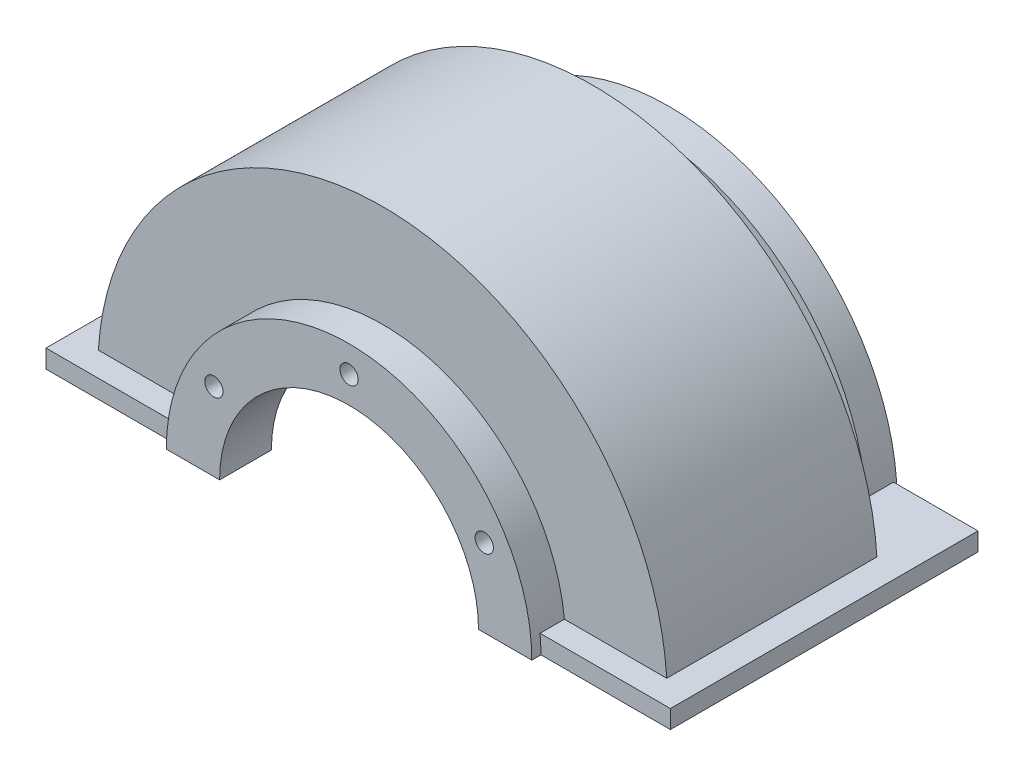
SolidWorks part; units mm, degrees
ref_plane "Front Plane" through (0, 0, 0) normal (0, 0, 1) x (1, 0, 0)
ref_plane "Top Plane" through (0, 0, 0) normal (0, 1, 0) x (1, 0, 0)
ref_plane "Right Plane" through (0, 0, 0) normal (1, 0, 0) x (0, 0, -1)
ref_plane "Plane1" through (0, 0, -358.693) normal (0, 0, -1) x (-1, 0, 0)
sketch "Sketch1" plane through (0, 0, -358.693) normal (0, 0, -1) x (-1, 0, 0)
  line L0 (-707.8452, 246.744) -> (-726.2306, 246.744)
  line L1 (-726.2306, 246.744) -> (-726.2306, 234.744)
  line L2 (-726.2306, 234.744) -> (-316.2306, 234.744)
  line L3 (-316.2306, 234.744) -> (-316.2306, 246.744)
  line L4 (-316.2306, 246.744) -> (-334.6161, 246.744)
  arc A0 (-334.6161, 246.744) -> (-707.8452, 246.744) centre (-521.2306, 234.744) ccw
  dimension "D1" = 187
  dimension "D2" = 18.3854
  dimension "D3" = 205
  dimension "D5" = 410
extrude "Boss-Extrude1" add sketch "Sketch1" against normal blind 202
sketch "Sketch2" plane through (0, 0, -156.693) normal (0, 0, 1) x (1, 0, 0)
  line L0 (640.6291, 246.744) -> (707.8452, 246.744)
  line L1 (334.6161, 246.744) -> (401.8322, 246.744)
  line L2 (316.2306, 234.744) -> (316.2306, 246.744) construction
  line L3 (316.2306, 246.744) -> (334.6161, 246.744) construction
  arc A0 (401.8322, 246.744) -> (640.6291, 246.744) centre (521.2306, 234.744) cw
  arc A1 (707.8452, 246.744) -> (334.6161, 246.744) centre (521.2306, 234.744) ccw
  dimension "D1" = 120
  dimension "D2" = 187
  dimension "D3" = 18.3854
  dimension "D4" = 85.6015
  dimension "D5" = 12
extrude "Cut-Extrude1" cut sketch "Sketch2" against normal blind 16
sketch "Sketch3" plane through (0, 0, -358.693) normal (0, 0, -1) x (-1, 0, 0)
  line L0 (-371.7114, 246.744) -> (-334.6161, 246.744)
  line L1 (-707.8452, 246.744) -> (-670.7499, 246.744)
  line L2 (-726.2306, 246.744) -> (-726.2306, 234.744) construction
  line L3 (-707.8452, 246.744) -> (-726.2306, 246.744) construction
  arc A0 (-670.7499, 246.744) -> (-371.7114, 246.744) centre (-521.2306, 234.744) cw
  arc A1 (-334.6161, 246.744) -> (-707.8452, 246.744) centre (-521.2306, 234.744) ccw
  dimension "D1" = 150
  dimension "D2" = 187
  dimension "D3" = 18.3854
  dimension "D4" = 55.4808
  dimension "D5" = 12
extrude "Cut-Extrude2" cut sketch "Sketch3" against normal blind 18
sketch "Sketch4" plane through (0, 0, -340.693) normal (0, 0, -1) x (-1, 0, 0)
  line L0 (-707.8452, 246.744) -> (-334.6161, 246.744)
  line L1 (-371.7114, 246.744) -> (-334.6161, 246.744) construction
  arc A0 (-334.6161, 246.744) -> (-707.8452, 246.744) centre (-521.2306, 234.744) ccw
  dimension "D1" = 187
  dimension "D2" = 149.5192
  dimension "D3" = 336.1338
  dimension "D4" = 12
extrude "Cut-Extrude3" cut sketch "Sketch4" against normal blind 30
sketch "Sketch5" plane through (0, 0, -358.693) normal (0, 0, -1) x (-1, 0, 0)
  line L0 (-371.2306, 234.744) -> (-671.2306, 234.744)
  line L1 (-726.2306, 246.744) -> (-726.2306, 234.744) construction
  line L2 (-670.7499, 246.744) -> (-726.2306, 246.744) construction
  arc A0 (-671.2306, 234.744) -> (-371.2306, 234.744) centre (-521.2306, 234.744) cw
  dimension "D1" = 150
  dimension "D2" = 205
  dimension "D3" = 12
extrude "Boss-Extrude2" add sketch "Sketch5" along normal blind 2
sketch "Sketch6" plane through (0, 0, -156.693) normal (0, 0, 1) x (1, 0, 0)
  line L0 (641.2306, 234.744) -> (401.2306, 234.744)
  line L1 (316.2306, 234.744) -> (316.2306, 246.744) construction
  line L2 (316.2306, 246.744) -> (401.8322, 246.744) construction
  arc A0 (401.2306, 234.744) -> (641.2306, 234.744) centre (521.2306, 234.744) cw
  dimension "D1" = 120
  dimension "D2" = 205
  dimension "D3" = 12
extrude "Boss-Extrude3" add sketch "Sketch6" along normal blind 6
sketch "Sketch7" plane through (0, 0, -340.693) normal (0, 0, 1) x (1, 0, 0)
  line L0 (619.5007, 246.744) -> (422.9606, 246.744)
  line L1 (670.7499, 246.744) -> (371.7114, 246.744) construction
  arc A0 (422.9606, 246.744) -> (619.5007, 246.744) centre (521.2306, 234.744) cw
  dimension "D1" = 99
  dimension "D2" = 51.2492
  dimension "D3" = 149.5192
  dimension "D4" = 12
extrude "Boss-Extrude4" add sketch "Sketch7" along normal blind 30
ref_plane "Plane2" through (0, 234.744, 0) normal (0, 1, 0) x (1, 0, 0)
sketch "Sketch8" plane through (0, 234.744, 0) normal (0, 1, 0) x (1, 0, 0)
  line L0 (606.2306, 360.693) -> (521.2306, 360.693)
  line L1 (521.2306, 360.693) -> (521.2306, 150.693)
  line L2 (521.2306, 150.693) -> (606.2306, 150.693)
  line L3 (606.2306, 150.693) -> (606.2306, 184.693)
  line L4 (606.2306, 184.693) -> (696.2306, 184.693)
  line L5 (696.2306, 184.693) -> (696.2306, 298.693)
  line L6 (696.2306, 298.693) -> (606.2306, 298.693)
  line L7 (606.2306, 298.693) -> (606.2306, 360.693)
  line L8 (521.2306, 360.693) -> (521.2306, 150.693) construction
  dimension "D1" = 85
  dimension "D2" = 175
  dimension "D3" = 34
  dimension "D4" = 148
  dimension "D5" = 210
revolve "Cut-Revolve1" cut sketch "Sketch8" angle 360 about L8
hole_wizard "Ø16.0 (16) diameter hole1" positions "Sketch10" profile "Sketch9" hole size "Ø16.0" standard "ANSI Metric"
sketch "Sketch10" plane through (0, 0, -340.693) normal (0, 0, 1) x (1, 0, 0)
  point P0 (421.6377, 292.244)
  point P1 (620.8236, 292.244)
sketch "Sketch9" plane through (421.6377, 292.244, -340.693) normal (1, 0, 0) x (0, -1, 0)
  line L0 (0, 0) -> (0, 20)
  line L1 (0, 20) -> (8, 20)
  line L2 (8, 20) -> (8, 0)
  line L5 (8, 0) -> (0, 0)
  line L11 (0, -6.35) -> (0, 107.95) construction
  dimension "通孔孔直径" = 16
  dimension "通孔孔深度" = 20
hole_wizard "Ø12.0 (12) diameter hole1" positions "Sketch12" profile "Sketch11" hole size "Ø12.0" standard "ANSI Metric"
sketch "Sketch12" plane through (0, 0, -150.693) normal (0, 0, 1) x (1, 0, 0)
  point P0 (521.2306, 337.244)
  point P1 (432.463, 285.994)
  point P2 (609.9982, 285.994)
sketch "Sketch11" plane through (521.2306, 337.244, -150.693) normal (1, 0, 0) x (0, -1, 0)
  line L0 (0, 0) -> (0, 34)
  line L1 (0, 34) -> (6, 34)
  line L2 (6, 34) -> (6, 0)
  line L5 (6, 0) -> (0, 0)
  line L11 (0, -6.35) -> (0, 107.95) construction
  dimension "通孔孔直径" = 12
  dimension "通孔孔深度" = 34
